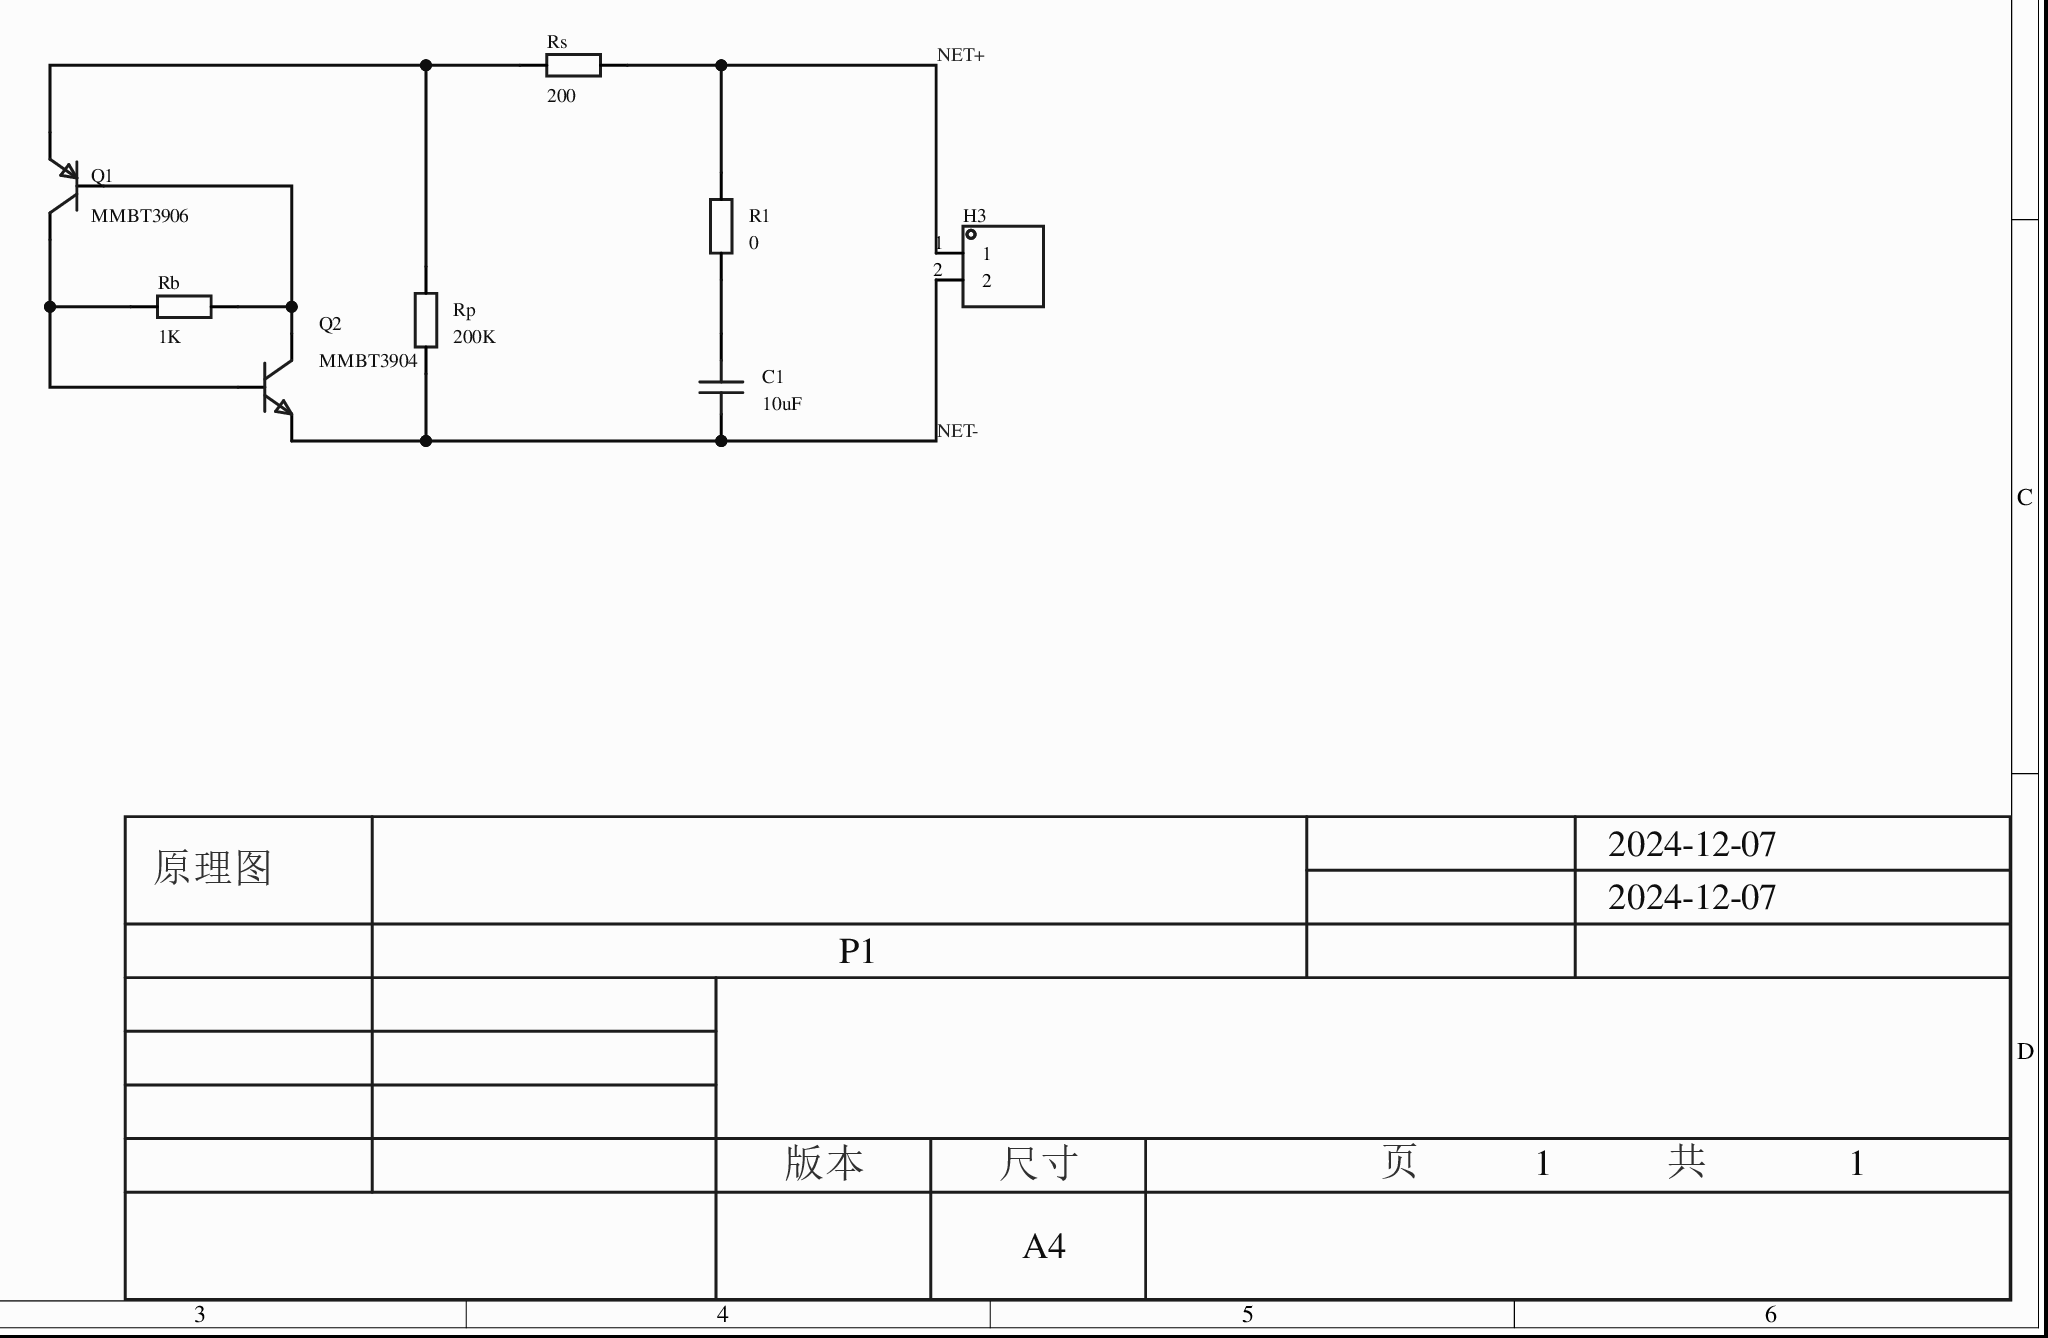
[diagram p0: MISC51453-3.schdoc]
# Altium project MISC51453-2.PrjPcb
1 sheet, 8 parts. Net scope: global (net labels, ports and power ports of the same name join across sheets).
Board file: MISC51453.pcbdoc

## Sheet MISC51453-3.schdoc
size 297 x 209 mm; Version: V1.0; @Project Name: MISC51453; @Page Count: 1; @Update Date: 2024-12-07; @Create Date: 2024-12-07; @Schematic Name: MISC51453; @Page No: 1; @Board Name: MISC51453; @Create Time: 12:51:08; @Update Time: 12:58:12

### Parts
C1  10uF  [C0402]
H3  (no value)  [HDR-TH_2P-P2.54-V-M-1]
Q1  MMBT3906  [SOT-23-3_L2.9-W1.3-P1.90-LS2.4-BR]
Q2  MMBT3904  [SOT-23-3_L2.9-W1.3-P1.90-LS2.4-BR]
R1  0  [R0402]
Rb  1K  [R0402]
Rp  200K  [R0402]
Rs  200  [R0402]

### Nets
NET+: H3.1 R1.2 Rs.2
NET-: C1.1 H3.2 Q2.2(E) Rp.1
NetC1_2: C1.2 R1.1
NetQ1_1: Q1.1(B) Q2.3(C) Rb.2
NetQ1_2: Q1.2(E) Rp.2 Rs.1
NetQ1_3: Q1.3(C) Q2.1(B) Rb.1

### Notes on the sheet
- 2024-12-07
- 原理图
- P1
- 版本
- 尺寸
- A4
- 页
- 1
- 共

### Library data of the parts
C1 = CAP_0402: ConvertToPcb: yes; SymbolName: CapAcitance; ModelId: 36a51122f27c49738f86b3bfa98863e0; ModelName: C0402_L1.0-W0.5-H0.5; ModelTransform: 39.37,19.685,0,0,0,0,0,0,0; Value: 10uF; Device: CAP_0402; AddInBom: yes; Supplier Footprint: 0402; FootprintName: C0402
H3 = HDR-M_2.54_1x2P: Symbol: 210S-1*2P L=11.6MMGold-plated black; ConvertToPcb: yes; ModelId: 79b2e9f2d70a4d68a1b7098f27c6d4c5; ModelName: HDR-M-2.54_1x2; ModelTransform: 200,100,0,0,0,0,0,0,-118.11; Device: HDR-M_2.54_1x2P; AddInBom: yes; SupplierPart: C124375; Supplier Footprint: 插件; FootprintName: HDR-TH_2P-P2.54-V-M-1
Q1 = MMBT3906_C18195368: Manufacturer: LJ(朗捷）; AddInBom: yes; ModelId: c62791f0466c4ae2a892c056b845b0ca; ModelName: SOT-23-3P_L2.9-W1.3-H1.0-LS2.4-P0.95; ModelTransform: 98.425,114.173,0,180,0,0,0.0005,-0.0005,0; Symbol: MMBT3906_C18195368; Device: MMBT3906_C18195368; LCSC Part Name: MMBT3906; SupplierPart: C18195368; ManufacturerPart: MMBT3906; Supplier Footprint: SOT-23; Datasheet: https://atta.szlcsc.com/upload/public/pdf/source/20230921/EBEA0117477174C76530FD120E2EA419.pdf; Supplier: LCSC; ConvertToPcb: yes; FootprintName: SOT-23-3_L2.9-W1.3-P1.90-LS2.4-BR
Q2 = MMBT3904: Manufacturer: Doeshare(德芯); Symbol: MMBT3904_C2931710; AddInBom: yes; ModelId: c62791f0466c4ae2a892c056b845b0ca; ModelName: SOT-23-3P_L2.9-W1.3-H1.0-LS2.4-P0.95; ModelTransform: 98.425,114.173,0,180,0,0,0.0005,-0.0005,0; Device: MMBT3904; LCSC Part Name: NPN 40V 200mA 100-300 SOT-23; SupplierPart: C2931710; ManufacturerPart: MMBT3904; Supplier Footprint: SOT-23; JLCPCB Part Class: 扩展库; Datasheet: https://atta.szlcsc.com/upload/public/pdf/source/20220104/14949413310F5EBD6E208F7B852FD0F0.pdf; Supplier: LCSC; ConvertToPcb: yes; FootprintName: SOT-23-3_L2.9-W1.3-P1.90-LS2.4-BR
R1 Rb Rp Rs = Res_0402: Symbol: 电阻; ConvertToPcb: yes; ModelId: 671aefced39d4c318694bba8bd8efd39; ModelName: R0402_L1.0-W0.5-H0.5; ModelTransform: 39.37,19.685,0,0,0,0,0,0.0005,0; Device: Res_0402; AddInBom: yes; Supplier Footprint: 0402; FootprintName: R0402
  R1: Value: 0
  Rb: Value: 1K
  Rp: Value: 200K
  Rs: Value: 200